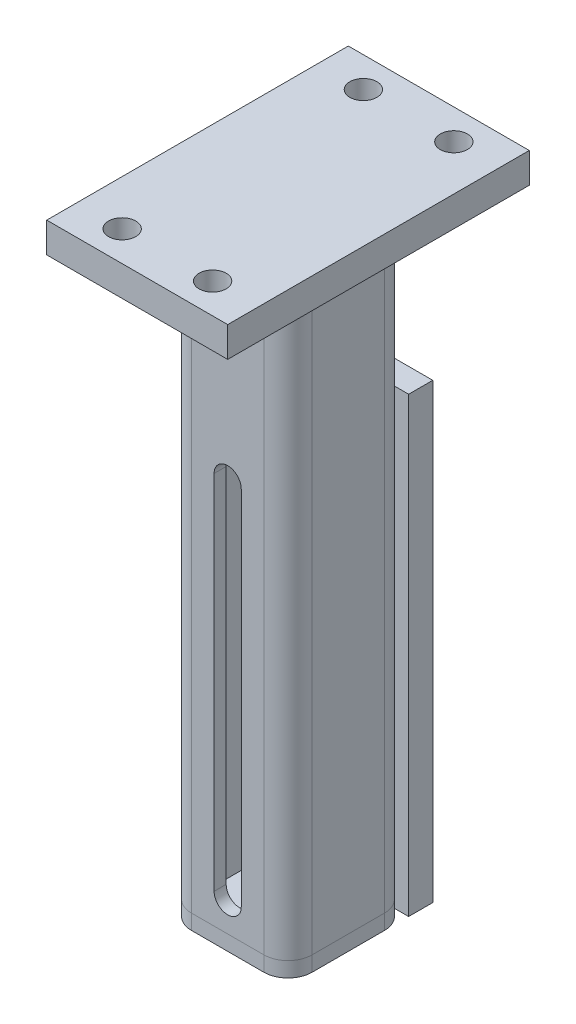
from build123d import *

# Parameters (mm, degrees)
F_40_X_40_X_4_0_1_DEPTH        = 200
SKETCH_4_W                     = 60
SKETCH_4_H                     = 100
EXTRUDE_1_DEPTH                = 10
END_CAP_1_THICKNESS            = 5
SKETCH_6_W                     = 4.5
SKETCH_6_H                     = 10
HOLE_WIZARD_9_0_9_1_AT_2_COUNT = 2
HOLE_WIZARD_9_0_9_1_AT_2_PITCH = 30
HOLE_WIZARD_9_0_9_1_AT_3_COUNT = 2
HOLE_WIZARD_9_0_9_1_AT_3_PITCH = 80
HOLE_WIZARD_9_0_9_1_AT_4_COUNT = 2
HOLE_WIZARD_9_0_9_1_AT_4_PITCH = 85.440037453
SKETCH_8_W                     = 40
SKETCH_8_H                     = 150
EXTRUDE_2_DEPTH                = 8
CUT_EXTRUDE_1_DEPTH            = 227.017698422


with BuildPart() as part:
    # Sketch1 → 方管 40 X 40 X 4.0(1) (new body)
    with BuildSketch(Plane(origin=(0, 0, 0), x_dir=(-1, 0, 0), z_dir=(0, 1, 0))):
        with BuildLine():
            Line((-12, -20), (12, -20))
            ThreePointArc((12, -20), (17.656854249, -17.656854249), (20, -12))
            Line((20, -12), (20, 12))
            ThreePointArc((20, 12), (17.656854249, 17.656854249), (12, 20))
            Line((12, 20), (-12, 20))
            ThreePointArc((-12, 20), (-17.656854249, 17.656854249), (-20, 12))
            Line((-20, 12), (-20, -12))
            ThreePointArc((-20, -12), (-17.656854249, -17.656854249), (-12, -20))
        make_face()
        with BuildLine():
            Line((-12, -16), (12, -16))
            ThreePointArc((12, -16), (14.828427125, -14.828427125), (16, -12))
            Line((16, -12), (16, 12))
            ThreePointArc((16, 12), (14.828427125, 14.828427125), (12, 16))
            Line((12, 16), (-12, 16))
            ThreePointArc((-12, 16), (-14.828427125, 14.828427125), (-16, 12))
            Line((-16, 12), (-16, -12))
            ThreePointArc((-16, -12), (-14.828427125, -14.828427125), (-12, -16))
        make_face(mode=Mode.SUBTRACT)
    extrude(amount=F_40_X_40_X_4_0_1_DEPTH)


with BuildPart() as body_2:
    # 草图4 → 凸台-拉伸1 (new body)
    with BuildSketch(Plane(origin=(0, 200, 0), x_dir=(1, 0, 0), z_dir=(0, 1, 0))):
        Rectangle(SKETCH_4_W, SKETCH_4_H)
    extrude(amount=EXTRUDE_1_DEPTH)

    # 草图6 → Ø9.0 (9) 直径孔1 (revolve, cut)
    with BuildSketch(Plane(origin=(15, 200, -40), x_dir=(0, 0, -1), z_dir=(1, 0, 0))):
        with Locations((2.25, 5)):
            Rectangle(SKETCH_6_W, SKETCH_6_H)
    hole_wizard_9_0_9_1 = revolve(axis=Axis((15, 193.65, -40), (0, 1, 0)), mode=Mode.SUBTRACT)

    # Ø9.0 (9) 直径孔1 at 2: Ø9.0 (9) 直径孔1 ×2
    with Locations(*[(-i * HOLE_WIZARD_9_0_9_1_AT_2_PITCH, 0, 0) for i in range(1, HOLE_WIZARD_9_0_9_1_AT_2_COUNT)]):
        add(hole_wizard_9_0_9_1, mode=Mode.SUBTRACT)

    # Ø9.0 (9) 直径孔1 at 3: Ø9.0 (9) 直径孔1 ×2
    with Locations(*[(0, 0, i * HOLE_WIZARD_9_0_9_1_AT_3_PITCH) for i in range(1, HOLE_WIZARD_9_0_9_1_AT_3_COUNT)]):
        add(hole_wizard_9_0_9_1, mode=Mode.SUBTRACT)

    # Ø9.0 (9) 直径孔1 at 4: Ø9.0 (9) 直径孔1 ×2
    with Locations(*[Vector(-0.3511234415883917, 0, 0.9363291775690445) * (i * HOLE_WIZARD_9_0_9_1_AT_4_PITCH) for i in range(1, HOLE_WIZARD_9_0_9_1_AT_4_COUNT)]):
        add(hole_wizard_9_0_9_1, mode=Mode.SUBTRACT)


with BuildPart() as body_3:
    # End Cap 1: an end cap: a plate 5.0 thick on the member's open end, its outline the end's outer outline
    end_cap_1_end = part.part.faces().sort_by_distance((16, 0, -16))[0]
    add(extrude(Face(end_cap_1_end.outer_wire()), amount=END_CAP_1_THICKNESS, dir=(0, 1, 0)))


with BuildPart() as part_1:
    add(part.part)

    # End Cap 1 3
    split(bisect_by=Plane(origin=(0, 5, 0), x_dir=(-1, 0, 0), z_dir=(0, 1, 0)), keep=Keep.TOP)


with BuildPart() as body_4:
    # 草图8 → 凸台-拉伸2 (new body)
    with BuildSketch(Plane(origin=(0, 0, -20), x_dir=(-1, 0, 0), z_dir=(0, 0, -1))):
        with Locations((0, 75)):
            Rectangle(SKETCH_8_W, SKETCH_8_H)
    extrude(amount=EXTRUDE_2_DEPTH)


with BuildPart() as cut_extrude_1_tool:
    # 草图9 → 切除-拉伸1 (new, through all)
    with BuildSketch(Plane(origin=(0, 0, -28), x_dir=(-1, 0, 0), z_dir=(0, 0, -1))):
        with BuildLine():
            Line((4.5, 135), (4.5, 15))
            ThreePointArc((4.5, 15), (0, 10.5), (-4.5, 15))
            Line((-4.5, 15), (-4.5, 135))
            ThreePointArc((-4.5, 135), (0, 139.5), (4.5, 135))
        make_face()
    extrude(amount=-CUT_EXTRUDE_1_DEPTH)


with BuildPart() as part_2:
    add(part_1.part)

    # 切除-拉伸1: cut by cut_extrude_1_tool
    add(cut_extrude_1_tool.part, mode=Mode.SUBTRACT)


with BuildPart() as body_4_1:
    add(body_4.part)

    # 切除-拉伸1: cut by cut_extrude_1_tool
    add(cut_extrude_1_tool.part, mode=Mode.SUBTRACT)


solid = Compound([body_2.part, body_3.part, part_2.part, body_4_1.part])
